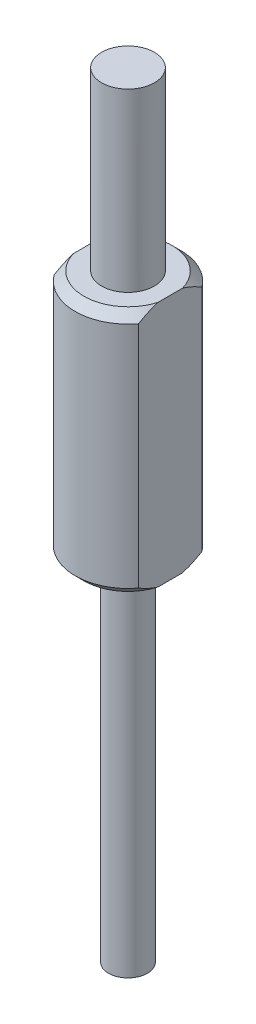
SolidWorks part; units mm, degrees
ref_plane "前视基准面" through (0, 0, 0) normal (0, 0, 1) x (1, 0, 0)
ref_plane "上视基准面" through (0, 0, 0) normal (0, 1, 0) x (1, 0, 0)
ref_plane "右视基准面" through (0, 0, 0) normal (1, 0, 0) x (0, 0, -1)
sketch "草图1" plane through (0, 0, 0) normal (0, 1, 0) x (1, 0, 0)
  circle A0 centre (0, 0) radius 1.5
  dimension "D1" = 3
extrude "凸台-拉伸1" add sketch "草图1" along normal blind 10
sketch "草图2" plane through (0, 0, 0) normal (0, -1, 0) x (1, 0, 0)
  circle A0 centre (0, 0) radius 3
  dimension "D1" = 6
extrude "M6X0.75P" add sketch "草图2" along normal blind 14
sketch "草图3" plane through (0, -14, 0) normal (0, -1, 0) x (1, 0, 0)
  circle A0 centre (0, 0) radius 1.1
  dimension "D1" = 2.2
extrude "凸台-拉伸3" add sketch "草图3" along normal blind 20
chamfer "倒角1" distance 0.5 angle 45 2 edges at (0, -14, -3) (0, 0, -3)
sketch "草图4" plane through (0, 10, 0) normal (0, 1, 0) x (1, 0, 0)
  line L0 (0, 0) -> (5.7708, 0) construction
  line L1 (4.4614, 3.7967) -> (2.4, 3.7967)
  line L2 (4.4614, 3.7967) -> (4.4614, -3.6919)
  line L3 (4.4614, -3.6919) -> (2.4, -3.6919)
  line L4 (2.4, 3.7967) -> (2.4, -3.6919)
  dimension "D1" = 2.4
extrude "切除-拉伸1" cut sketch "草图4" against normal through all
mirror "镜向1" about plane through (0, 0, 0) normal (1, 0, 0) of "切除-拉伸1"
